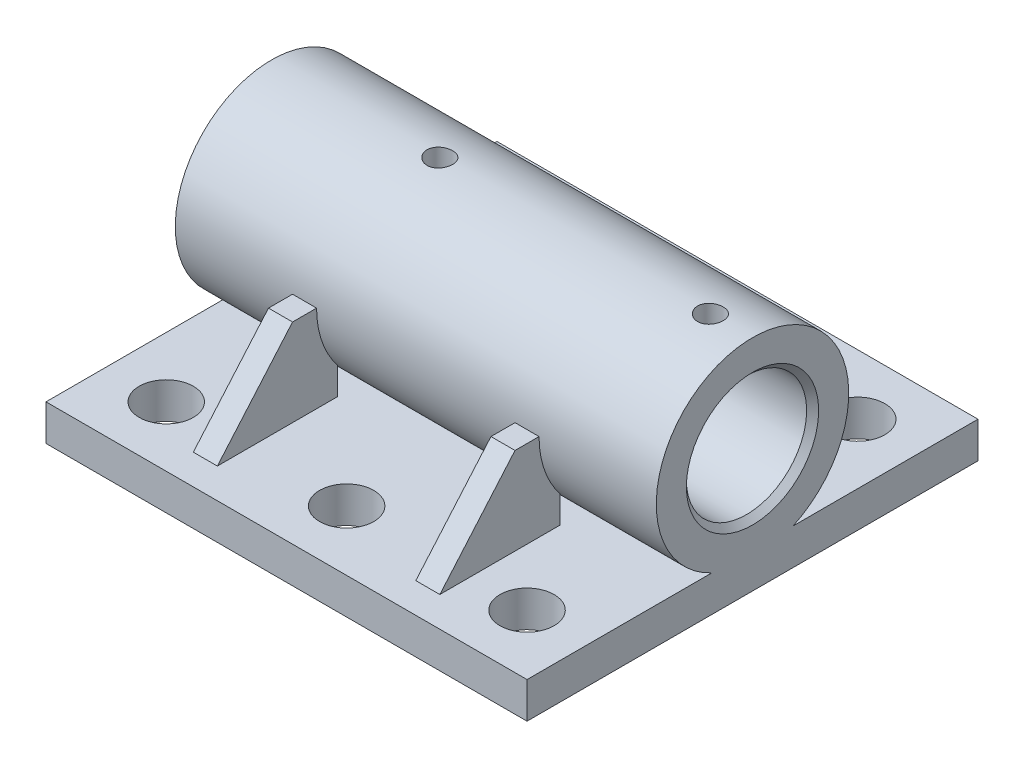
from build123d import *

# Parameters (mm, degrees)
SKETCH_1_W                   = 160
SKETCH_1_H                   = 150
SKETCH_1_R                   = 9
EXTRUDE_1_DEPTH              = 12
EXTRUDE_START                = 33
EXTRUDE_2_DEPTH              = 8
HOLE_WIZARD_M10_1_AT_2_COUNT = 2
HOLE_WIZARD_M10_1_AT_2_PITCH = 90
CHAMFER_1_SIZE               = 1
CHAMFER_2_SIZE               = 2


with BuildPart() as part:
    # 草图1 → 凸台-拉伸1 (new body)
    with BuildSketch(Plane(origin=(0, 0, 0), x_dir=(1, 0, 0), z_dir=(0, 1, 0))):
        Rectangle(SKETCH_1_W, SKETCH_1_H)
        with Locations(Location((-60, -55, 0), (0, 0, 270))):
            Circle(SKETCH_1_R, mode=Mode.SUBTRACT)
        with Locations(Location((0, -55, 0), (0, 0, 270))):
            Circle(SKETCH_1_R, mode=Mode.SUBTRACT)
        with Locations(Location((60, -55, 0), (0, 0, 270))):
            Circle(SKETCH_1_R, mode=Mode.SUBTRACT)
        with Locations(Location((0, 55, 0), (0, 0, 270))):
            Circle(SKETCH_1_R, mode=Mode.SUBTRACT)
        with Locations(Location((60, 55, 0), (0, 0, 270))):
            Circle(SKETCH_1_R, mode=Mode.SUBTRACT)
        with Locations(Location((-60, 55, 0), (0, 0, 270))):
            Circle(SKETCH_1_R, mode=Mode.SUBTRACT)
    extrude(amount=EXTRUDE_1_DEPTH)

    # 草图2 → 旋转1 (revolve)
    with BuildSketch(Plane.XY, mode=Mode.PRIVATE) as revolve_1_sk:
        Polygon((-80, 56), (-60, 56), (-60, 64), (40, 64), (40, 61), (80, 61), (80, 73), (-80, 73), align=None)
    revolve(revolve_1_sk.sketch.rotate(Axis((-77.946721126, 41, 0), (1, 0, 0)), 90), axis=Axis((-77.946721126, 41, 0), (1, 0, 0)))

    # 草图6 → M10 螺纹孔1 (revolve, cut)
    with BuildSketch(Plane(origin=(-24, 73, 0), x_dir=(0, 0, 1), z_dir=(1, 0, 0))):
        Polygon((0, 0), (0, 30.053657631), (4.25, 27.5), (4.25, 0), align=None)
    hole_wizard_m10_1 = revolve(axis=Axis((-24, 79.35, 0), (0, -1, 0)), mode=Mode.SUBTRACT)

    # M10 螺纹孔1 at 2: M10 螺纹孔1 ×2
    with Locations(*[(i * HOLE_WIZARD_M10_1_AT_2_PITCH, 0, 0) for i in range(1, HOLE_WIZARD_M10_1_AT_2_COUNT)]):
        add(hole_wizard_m10_1, mode=Mode.SUBTRACT)

    # 倒角1
    chamfer_1_edges = [part.edges().sort_by_distance(p)[0] for p in [
        (-80, 41, -15),
    ]]
    chamfer(chamfer_1_edges, length=CHAMFER_1_SIZE)

    # 倒角2
    chamfer_2_edges = [part.edges().sort_by_distance(p)[0] for p in [
        (80, 41, -20),
    ]]
    chamfer(chamfer_2_edges, length=CHAMFER_2_SIZE)


with BuildPart() as body_2:
    # 草图4 → 凸台-拉伸2 (new body)
    with BuildSketch(Plane(origin=(0, 0, 0), x_dir=(0, 0, -1), z_dir=(1, 0, 0)).offset(EXTRUDE_START)):
        with BuildLine():
            Line((-32, 41), (-40, 41))
            Line((-40, 41), (-65, 12))
            Line((-65, 12), (-25, 12))
            Line((-25, 12), (-25, 21.025015645))
            ThreePointArc((-25, 21.025015645), (-30.199337741, 30.416994756), (-32, 41))
        make_face()
    extrude(amount=EXTRUDE_2_DEPTH)


with BuildPart() as body_3:
    # 镜向1: mirrored copy
    add(body_2.part.mirror(Plane.XY))


with BuildPart() as body_4:
    # 镜向2: mirrored copy
    add(body_3.part.mirror(Plane(origin=(0, 0, 0), x_dir=(0, 0, 1), z_dir=(1, 0, 0))))


with BuildPart() as body_5:
    # Mirror 2 2: mirrored copy
    add(body_2.part.mirror(Plane(origin=(0, 0, 0), x_dir=(0, 0, 1), z_dir=(1, 0, 0))))


solid = Compound([part.part, body_2.part, body_3.part, body_4.part, body_5.part])
